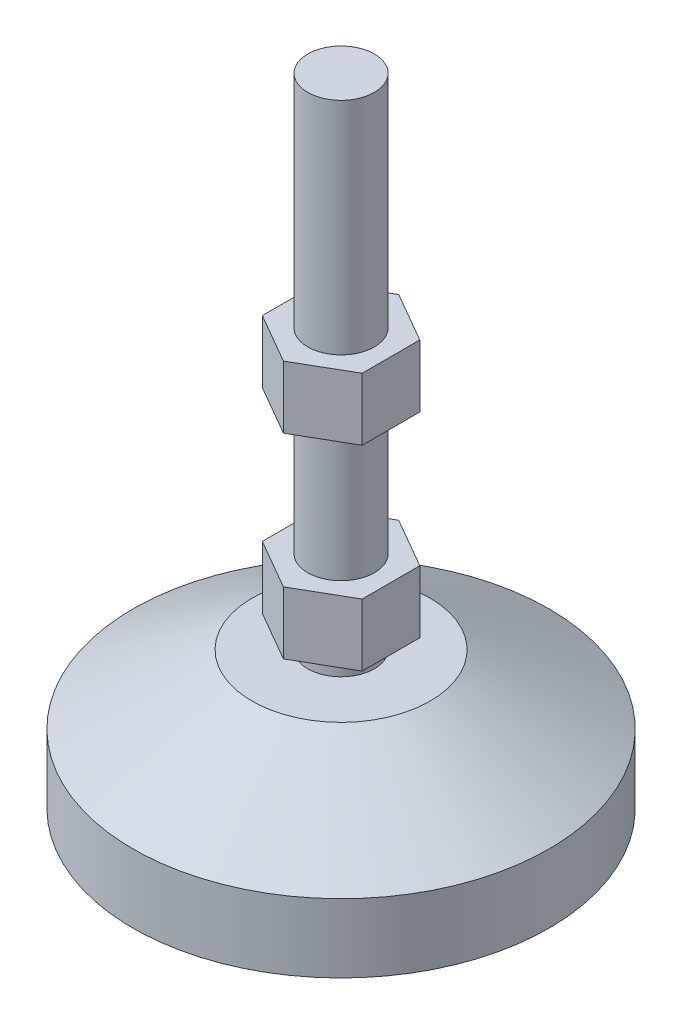
from build123d import *

# Parameters (mm, degrees)
EXTRUDE_START        = 5
EXTRUDE_1_DEPTH      = 15
EXTRUDE_2_DEPTH      = 100
EXTRUDE_2_DEPTH_BACK = 53
SKETCH_3_R           = 8
EXTRUDE_START_2      = 100
EXTRUDE_3_DEPTH      = 15


with BuildPart() as part:
    # 草图1 → 旋转1 (revolve)
    with BuildSketch(Plane.XY, mode=Mode.PRIVATE) as revolve_1_sk:
        Polygon((0, 0), (50, 0), (50, 16.5), (21.421161675, 33), (0, 33), align=None)
    revolve(revolve_1_sk.sketch.rotate(Axis((0, 0, 0), (0, 1, 0)), 90), axis=Axis((0, 0, 0), (0, 1, 0)))

    # 草图3 → 凸台-拉伸2 (add, two sides: drawn at the far end of the back side and taken through both)
    with BuildSketch(Plane(origin=(0, 53, 0), x_dir=(1, 0, 0), z_dir=(0, 1, 0)).offset(-EXTRUDE_2_DEPTH_BACK)):
        with Locations(Location((0, 0, 0), (0, 0, 270))):
            Circle(SKETCH_3_R)
    extrude(amount=EXTRUDE_2_DEPTH + EXTRUDE_2_DEPTH_BACK)

    # 草图4 → 凸台-拉伸3 (add)
    with BuildSketch(Plane(origin=(0, 0, 0), x_dir=(1, 0, 0), z_dir=(0, 1, 0)).offset(EXTRUDE_START_2)):
        Polygon((0, -13.856406461), (12, -6.92820323), (12, 6.92820323), (0, 13.856406461), (-12, 6.92820323), (-12, -6.92820323), align=None)
    extrude(amount=-EXTRUDE_3_DEPTH)


with BuildPart() as body_2:
    # 草图2 → 凸台-拉伸1 (new body)
    with BuildSketch(Plane(origin=(0, 33, 0), x_dir=(1, 0, 0), z_dir=(0, 1, 0)).offset(EXTRUDE_START)):
        Polygon((12, -6.92820323), (12, 6.92820323), (0, 13.856406461), (-12, 6.92820323), (-12, -6.92820323), (0, -13.856406461), align=None)
    extrude(amount=EXTRUDE_1_DEPTH)


solid = Compound([part.part, body_2.part])
